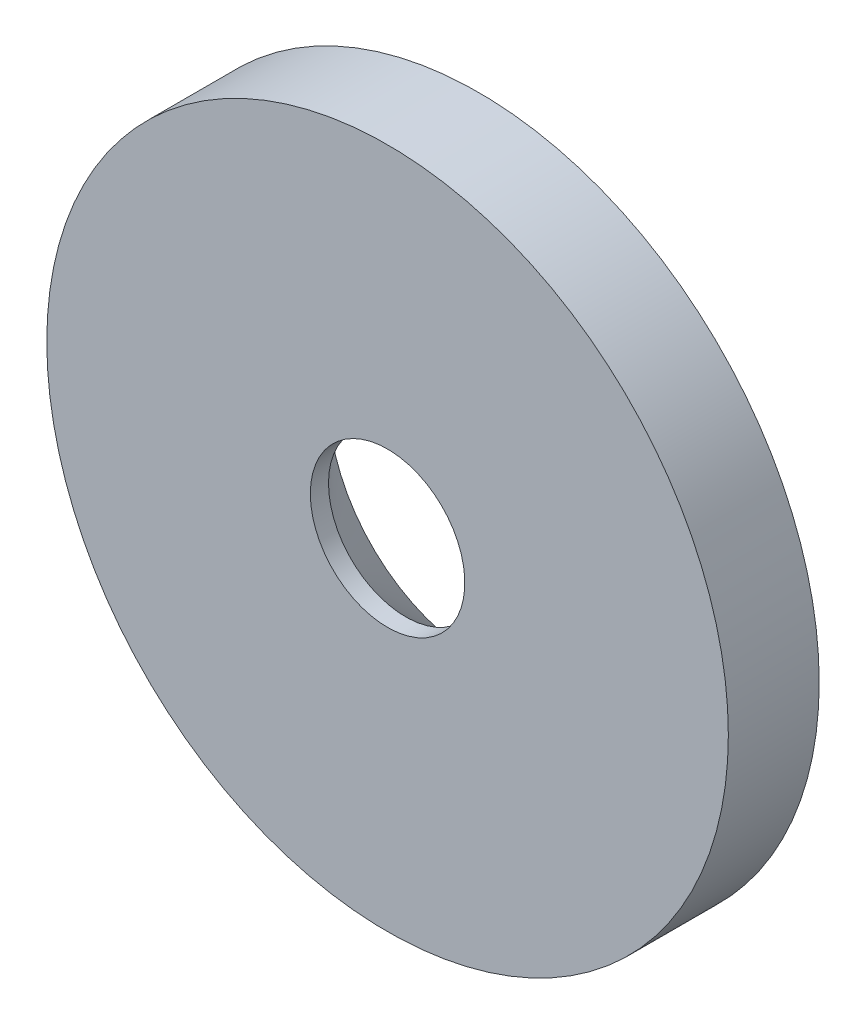
from build123d import *

# Parameters (mm, degrees)
SKETCH_1_R      = 7.5
SKETCH_1_R_2    = 1
EXTRUDE_1_DEPTH = 2


with BuildPart() as part:
    # 草图1 → 凸台-拉伸1 (new body)
    with BuildSketch(Plane.XY):
        Circle(SKETCH_1_R)
        Circle(SKETCH_1_R_2, mode=Mode.SUBTRACT)
    extrude(amount=EXTRUDE_1_DEPTH)

    # 草图5 → M3 开槽沉头木螺钉的锥形沉头孔1 (revolve, cut)
    with BuildSketch(Plane.YZ):
        Polygon((0, 0), (0, 2), (1.7, 2), (1.7, 1.6), (3.3, 0), align=None)
    revolve(axis=Axis((0, 0, -6.35), (0, 0, 1)), mode=Mode.SUBTRACT)


solid = part.part
